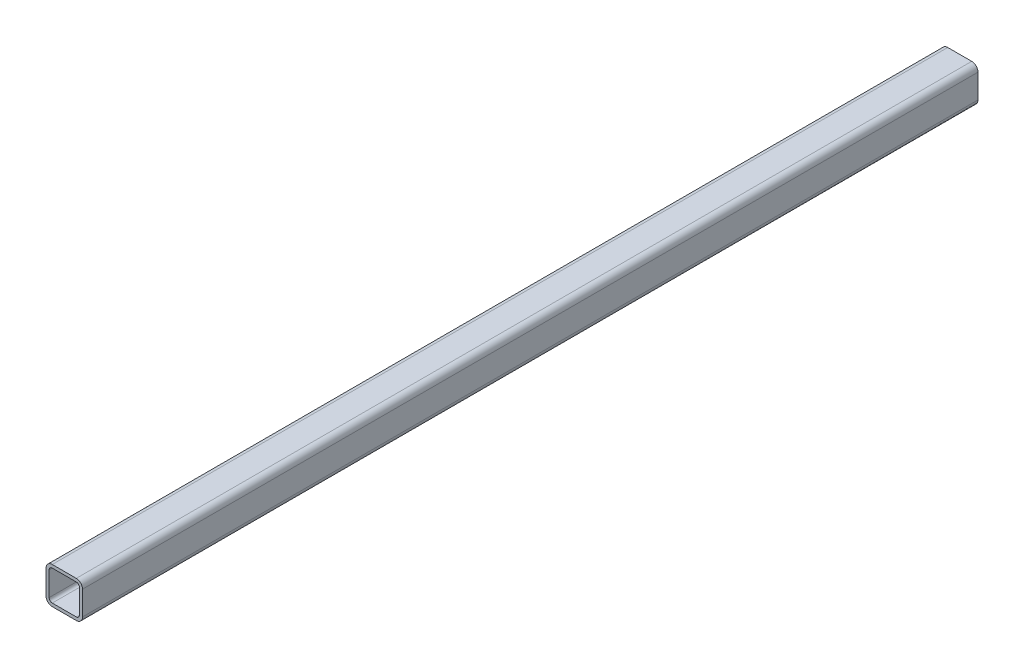
from build123d import *

# Parameters (mm, degrees)
BOSS_EXTRUDE1_DEPTH = 1716


with BuildPart() as part:
    # Sketch1 → Boss-Extrude1 (new body)
    with BuildSketch(Plane.XY):
        with BuildLine():
            Line((12, 0), (58, 0))
            ThreePointArc((58, 0), (66.485281374, 3.514718626), (70, 12))
            Line((70, 12), (70, 58))
            ThreePointArc((70, 58), (66.485281374, 66.485281374), (58, 70))
            Line((58, 70), (12, 70))
            ThreePointArc((12, 70), (3.514718626, 66.485281374), (0, 58))
            Line((0, 58), (0, 12))
            ThreePointArc((0, 12), (3.514718626, 3.514718626), (12, 0))
        make_face()
        with BuildLine():
            Line((12, 6), (58, 6))
            ThreePointArc((58, 6), (62.242640687, 7.757359313), (64, 12))
            Line((64, 12), (64, 58))
            ThreePointArc((64, 58), (62.242640687, 62.242640687), (58, 64))
            Line((58, 64), (12, 64))
            ThreePointArc((12, 64), (7.757359313, 62.242640687), (6, 58))
            Line((6, 58), (6, 12))
            ThreePointArc((6, 12), (7.757359313, 7.757359313), (12, 6))
        make_face(mode=Mode.SUBTRACT)
    extrude(amount=BOSS_EXTRUDE1_DEPTH)


solid = part.part
